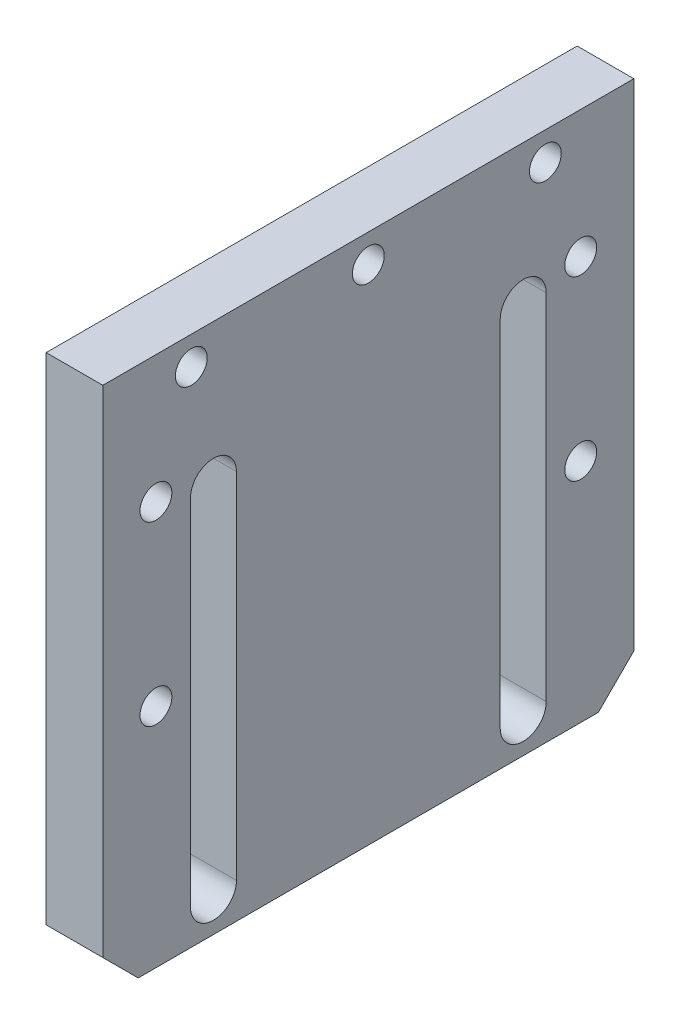
from build123d import *

# Parameters (mm, degrees)
SKETCH_1_W                = 150
SKETCH_1_H                = 150
EXTRUDE_1_DEPTH           = 16
CUT_EXTRUDE_1_DEPTH       = 108.266024444
HOLE_WIZARD_1_D           = 9
HOLE_WIZARD_1_DEPTH       = 29.25
HOLE_WIZARD_1_CBORE_D     = 15
HOLE_WIZARD_1_CBORE_DEPTH = 9
HOLE_WIZARD_1_TIP         = 2.703872786
HOLE_WIZARD_2_D           = 9
HOLE_WIZARD_2_DEPTH       = 29.25
HOLE_WIZARD_2_CBORE_D     = 15
HOLE_WIZARD_2_CBORE_DEPTH = 9
HOLE_WIZARD_2_TIP         = 2.703872786
CHAMFER_1_SIZE            = 10


with BuildPart() as part:
    # 草图1 → 凸台-拉伸1 (new body)
    with BuildSketch(Plane(origin=(0, 0, 0), x_dir=(0, 0, -1), z_dir=(1, 0, 0))):
        Rectangle(SKETCH_1_W, SKETCH_1_H)
    extrude(amount=EXTRUDE_1_DEPTH)

    # 草图3 → 切除-拉伸1 (cut, through all)
    with BuildSketch(Plane(origin=(16, 0, 0), x_dir=(0, 0, -1), z_dir=(1, 0, 0))):
        with BuildLine():
            Line((-37.253402877, 35), (-37.253402877, -65))
            ThreePointArc((-37.253402877, -65), (-43.753402877, -71.5), (-50.253402877, -65))
            Line((-50.253402877, -65), (-50.253402877, 35))
            ThreePointArc((-50.253402877, 35), (-43.753402877, 41.5), (-37.253402877, 35))
        make_face()
        with BuildLine():
            Line((50.253402877, 35), (50.253402877, -65))
            ThreePointArc((50.253402877, -65), (43.753402877, -71.5), (37.253402877, -65))
            Line((37.253402877, -65), (37.253402877, 35))
            ThreePointArc((37.253402877, 35), (43.753402877, 41.5), (50.253402877, 35))
        make_face()
    extrude(amount=-CUT_EXTRUDE_1_DEPTH, mode=Mode.SUBTRACT)

    # 打孔尺寸(%根据)内六角圆柱头螺钉的类型1
    with Locations(Plane.ZY):
        with Locations((-50, 67), (0, 67), (50, 67)):
            CounterBoreHole(HOLE_WIZARD_1_D / 2, HOLE_WIZARD_1_CBORE_D / 2, HOLE_WIZARD_1_CBORE_DEPTH, depth=HOLE_WIZARD_1_DEPTH)
            with Locations((0, 0, -(HOLE_WIZARD_1_DEPTH + HOLE_WIZARD_1_TIP / 2))):  # 118° drill point
                Cone(0, HOLE_WIZARD_1_D / 2, HOLE_WIZARD_1_TIP, mode=Mode.SUBTRACT)

    # 打孔尺寸(%根据)内六角圆柱头螺钉的类型2
    with Locations(Plane.ZY):
        with Locations((-60, 39), (-60, -11), (60, 39), (60, -11)):
            CounterBoreHole(HOLE_WIZARD_2_D / 2, HOLE_WIZARD_2_CBORE_D / 2, HOLE_WIZARD_2_CBORE_DEPTH, depth=HOLE_WIZARD_2_DEPTH)
            with Locations((0, 0, -(HOLE_WIZARD_2_DEPTH + HOLE_WIZARD_2_TIP / 2))):  # 118° drill point
                Cone(0, HOLE_WIZARD_2_D / 2, HOLE_WIZARD_2_TIP, mode=Mode.SUBTRACT)

    # 倒角1
    chamfer_1_edges = [part.edges().sort_by_distance(p)[0] for p in [
        (8, -75, -75),
        (8, -75, 75),
    ]]
    chamfer(chamfer_1_edges, length=CHAMFER_1_SIZE)


solid = part.part
